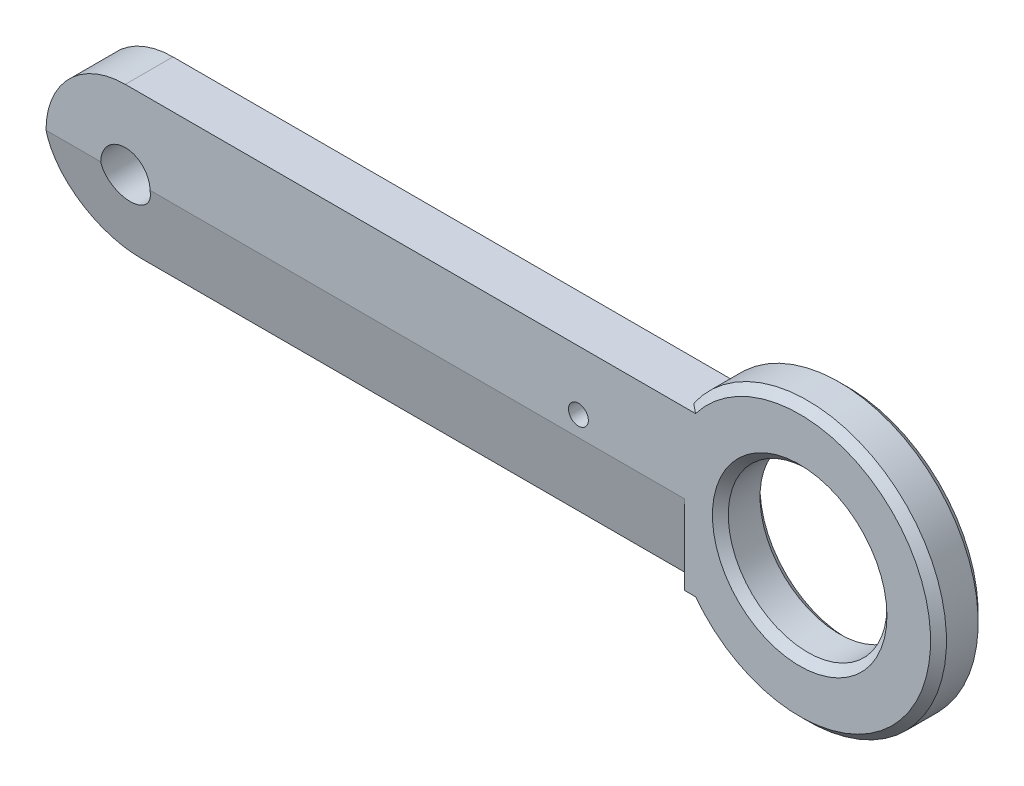
SolidWorks part; units mm, degrees
material "SUS304"
ref_plane "前视基准面" through (0, 0, 0) normal (0, 0, 1) x (1, 0, 0)
ref_plane "上视基准面" through (0, 0, 0) normal (0, 1, 0) x (1, 0, 0)
ref_plane "右视基准面" through (0, 0, 0) normal (1, 0, 0) x (0, 0, -1)
sketch "草图6" plane through (0, 0, 0) normal (0, 0, 1) x (1, 0, 0)
  line L0 (-42.5, 0) -> (42.5, 0) construction
  line L5 (-42.5, 10) -> (42.5, 10)
  line L6 (-42.5, -10) -> (42.5, -10)
  arc A0 (-42.5, 10) -> (-42.5, -10) centre (-42.5, 0) ccw
  arc A1 (42.5, -10) -> (42.5, 10) centre (42.5, 0) ccw
  circle A2 centre (42.5, 0) radius 17.5
  point P2 (0, 0)
  dimension "D2" = 10
  dimension "D3" = 35
  dimension "D1" = 85
extrude "凸台-拉伸3" add sketch "草图6" along normal blind 6
sketch "草图7" plane through (0, 0, 0) normal (0, 0, -1) x (-1, 0, 0)
  circle A0 centre (-42.5, 0) radius 10
  dimension "D1" = 20
extrude "切除-拉伸1" cut sketch "草图7" against normal blind 10
sketch "草图8" plane through (0, 0, 0) normal (0, 0, -1) x (-1, 0, 0)
  circle A0 centre (42.5, 0) radius 3.1
  dimension "D1" = 6.2
extrude "切除-拉伸2" cut sketch "草图8" against normal blind 10
ref_plane "基准面1" through (28, 0, 0) normal (1, 0, 0) x (0, 0, -1)
sketch "草图9" plane through (28, 0, 0) normal (1, 0, 0) x (0, 0, -1)
  line L0 (-4, -10) -> (-6, 0)
  line L1 (-6, -10) -> (0, -10) construction
  line L2 (-6, 17.5) -> (-6, -17.5) construction
  line L3 (-6, 0) -> (-6, -10)
  line L4 (-6, -10) -> (-4, -10)
  line L5 (-2, -10) -> (0, 0)
  line L7 (0, 0) -> (0, -10)
  line L8 (0, -10) -> (-2, -10)
  line L9 (-6, 0) -> (0, 0) construction
  dimension "D1" = 2
  dimension "D2" = 10
extrude "切除-拉伸3" cut sketch "草图9" against normal through all
chamfer "倒角1" distance 1 angle 45 4 edges at (52.5, 0, 6) (60, 0, 6) (60, 0, 0) (32.5, 0, 0)
hole_wizard "M3 螺纹孔1" positions "草图10" profile "草图11" tap size "M3" standard "ISO"
sketch "草图10" plane through (0, 0, 0) normal (0, 0, -1) x (-1, 0, 0)
  point P0 (-14.6118, 2.5)
sketch "草图11" plane through (14.6118, 2.5, 0) normal (1, 0, 0) x (0, 1, 0)
  line L0 (0, 0) -> (0, 9.2511)
  line L1 (0, 9.2511) -> (1.25, 8.5)
  line L2 (1.25, 8.5) -> (1.25, 0)
  line L5 (1.25, 0) -> (0, 0)
  line L10 (0, 9.2511) -> (-1.25, 8.5) construction
  line L11 (0, -6.35) -> (0, 107.95) construction
  dimension "螺纹孔钻头直径" = 2.5
  dimension "螺纹孔钻头深度" = 8.5
  dimension "导头角度" = 118
cosmetic thread "孔螺蚊线1" parameters "D1"=6, "D2"=3
